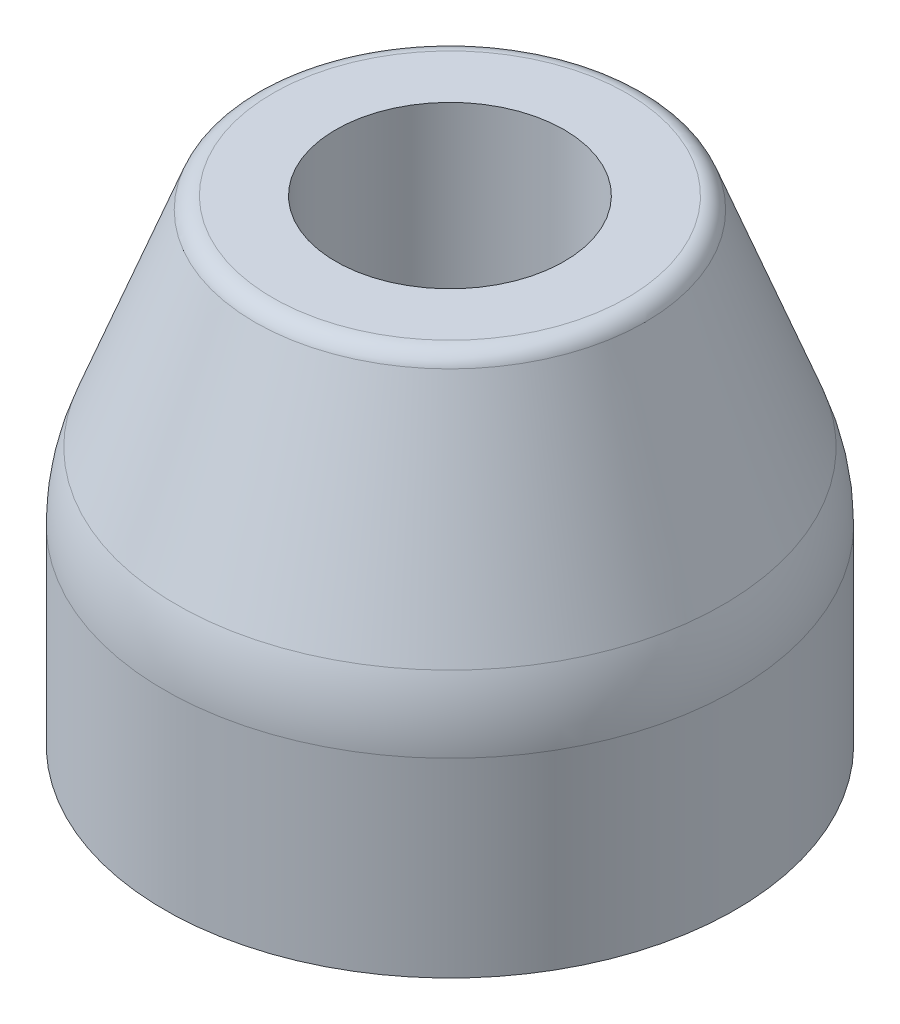
SolidWorks part; units mm, degrees
ref_plane "Front Plane" through (0, 0, 0) normal (0, 0, 1) x (1, 0, 0)
ref_plane "Top Plane" through (0, 0, 0) normal (0, 1, 0) x (1, 0, 0)
ref_plane "Right Plane" through (0, 0, 0) normal (1, 0, 0) x (0, 0, -1)
sketch "Sketch1" plane through (0, 0, 0) normal (0, 0, 1) x (1, 0, 0)
  line L0 (4, 0) -> (4, 11)
  line L1 (6, 25) -> (9.3101, 25)
  line L2 (10.2449, 24.3551) -> (14.3485, 13.5505)
  line L3 (15, 10) -> (15, 0)
  line L4 (15, 0) -> (4, 0)
  line L5 (6, 25) -> (6, 11)
  line L6 (4, 11) -> (6, 11)
  line L7 (0, 0) -> (0, 35.8691) construction
  arc A0 (14.3485, 13.5505) -> (15, 10) centre (5, 10) cw
  arc A1 (10.2449, 24.3551) -> (9.3101, 25) centre (9.3101, 24) ccw
  point P9 (15, 11.835)
  point P14 (10, 25)
  dimension "D5" = 10
  dimension "D6" = 15
  dimension "D9" = 1
  dimension "D1" = 4
  dimension "D2" = 6
  dimension "D3" = 25
  dimension "D4" = 14
  dimension "D7" = 10
  dimension "D8" = 10
revolve "Revolve1" add sketch "Sketch1" angle 360 about L7
